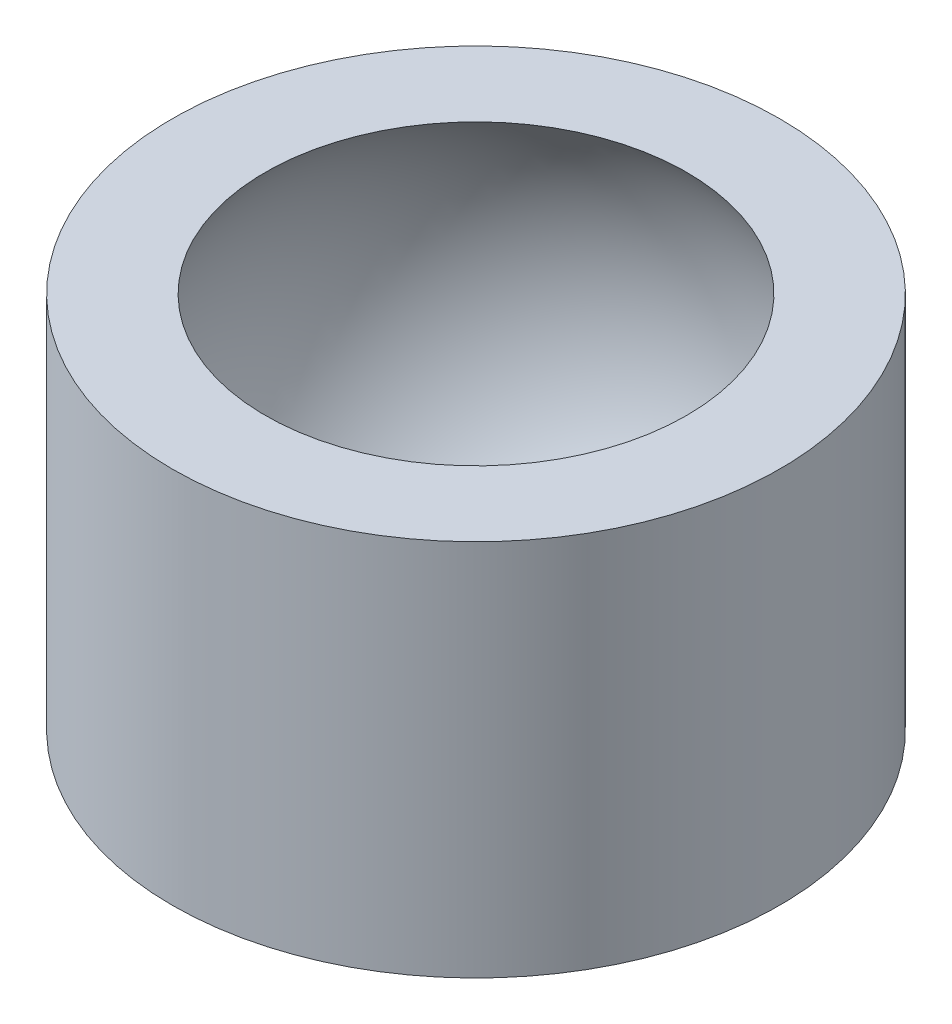
SolidWorks part; units mm, degrees
material "普通碳钢"
ref_plane "前视" through (0, 0, 0) normal (0, 0, 1) x (1, 0, 0)
ref_plane "上视" through (0, 0, 0) normal (0, 1, 0) x (1, 0, 0)
ref_plane "右视" through (0, 0, 0) normal (1, 0, 0) x (0, 0, -1)
sketch "草图1" plane through (0, 0, 0) normal (0, 0, 1) x (1, 0, 0)
  line L0 (-41.0431, 0) -> (41.3464, 0) construction
  line L1 (0, 29.923) -> (0, -26.587) construction
  line L2 (15.6125, 12.5) -> (22.5, 12.5)
  line L3 (22.5, 12.5) -> (22.5, -15.5)
  line L4 (22.5, -15.5) -> (19.3, -15.5)
  line L6 (19.3, -15.5) -> (15.6125, -12.5)
  arc A1 (15.6125, -12.5) -> (15.6125, 12.5) centre (0, 0) ccw
  dimension "D1" = 22.5
  dimension "D2" = 12.5
  dimension "D3" = 15.5
  dimension "D4" = 19.3
revolve "旋转1" add sketch "草图1" angle 360 about L1
